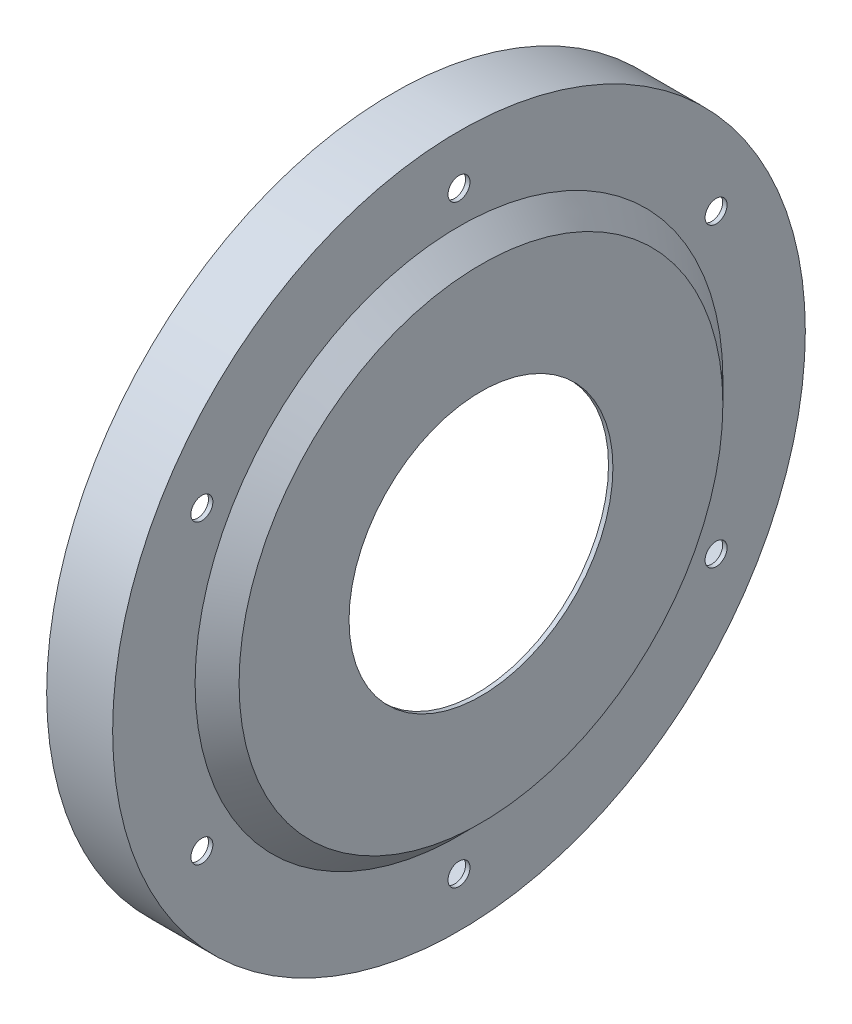
SolidWorks part; units mm, degrees
ref_plane "Front Plane" through (0, 0, 0) normal (0, 0, 1) x (1, 0, 0)
ref_plane "Top Plane" through (0, 0, 0) normal (0, 1, 0) x (1, 0, 0)
ref_plane "Right Plane" through (0, 0, 0) normal (1, 0, 0) x (0, 0, -1)
other "Configuration Table"
sketch "Sketch1" plane through (0, 0, 0) normal (0, 1, 0) x (1, 0, 0)
  line L0 (0, 0) -> (60, 0) construction
  line L1 (0, 0) -> (0, 157.5)
  line L2 (0, 157.5) -> (30, 157.5)
  line L3 (30, 157.5) -> (30, 120)
  line L4 (30, 120) -> (40, 110)
  line L5 (40, 110) -> (40, 0)
  line L6 (0, 0) -> (40, 0)
  dimension "D1" = 30
  dimension "D2" = 40
  dimension "D3" = 315
  dimension "D4" = 240
  dimension "D5" = 45
revolve "Revolve1" add sketch "Sketch1" angle 360 about L0
shell "Shell1" thickness 2
sketch "Sketch2" plane through (40, 0, 0) normal (1, 0, 0) x (0, 0, -1)
  circle A0 centre (0, 0) radius 60
  dimension "D1" = 120
extrude "Cut-Extrude1" cut sketch "Sketch2" against normal blind 50
sketch "Sketch3" plane through (30, 0, 0) normal (1, 0, 0) x (0, 0, -1)
  circle A0 centre (0, 0) radius 135 construction
  circle A1 centre (0, 135) radius 5
  circle A2 centre (116.9134, 67.5) radius 5
  circle A3 centre (116.9134, -67.5) radius 5
  circle A4 centre (0, -135) radius 5
  circle A5 centre (-116.9134, -67.5) radius 5
  circle A6 centre (-116.9134, 67.5) radius 5
  point P18 (0, 0)
  dimension "D1" = 270
  dimension "D2" = 10
  dimension "D3" = 6
extrude "Cut-Extrude2" cut sketch "Sketch3" against normal blind 50
